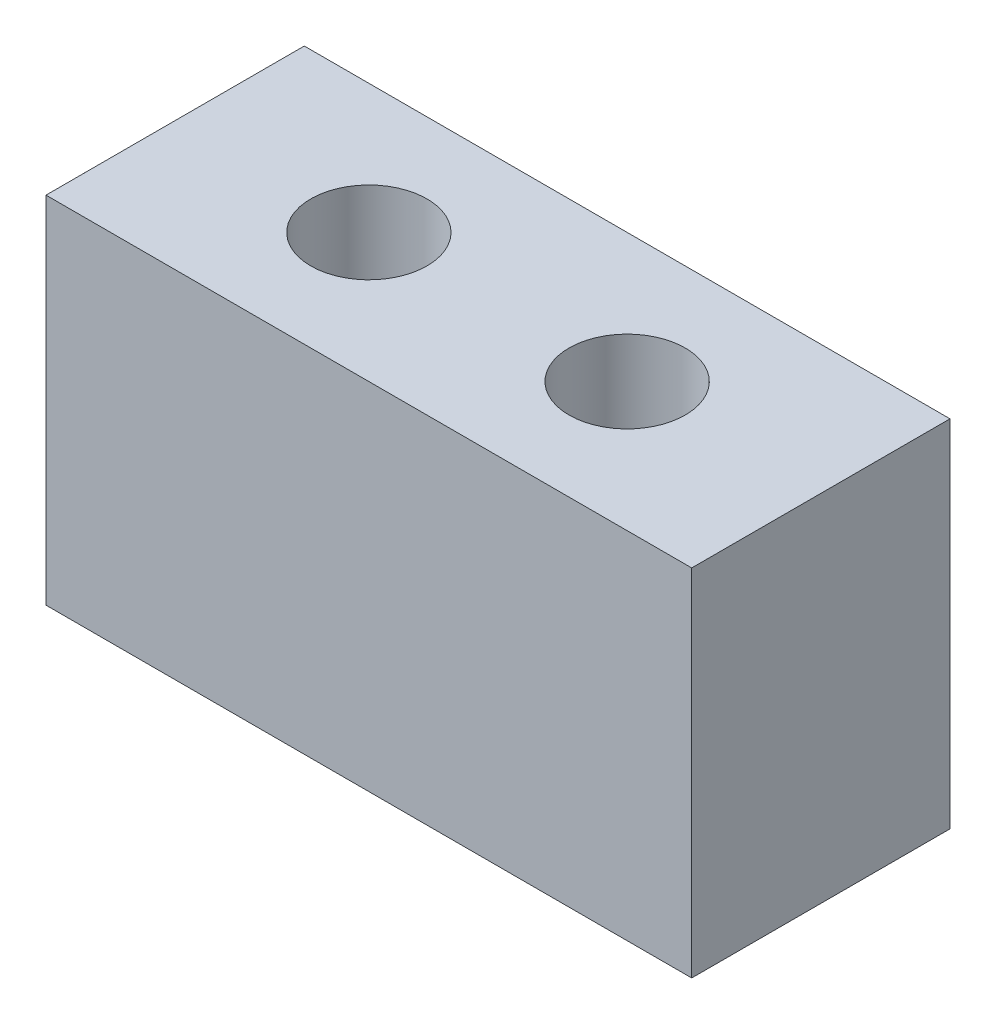
SolidWorks part; units mm, degrees
ref_plane "Front Plane" through (0, 0, 0) normal (0, 0, 1) x (1, 0, 0)
ref_plane "Top Plane" through (0, 0, 0) normal (0, 1, 0) x (1, 0, 0)
ref_plane "Right Plane" through (0, 0, 0) normal (1, 0, 0) x (0, 0, -1)
sketch "Sketch1" plane through (0, 0, 0) normal (0, 1, 0) x (1, 0, 0)
  line L1 (-50, -20) -> (50, -20)
  line L2 (-50, -20) -> (-50, 20)
  line L3 (-50, 20) -> (50, 20)
  line L4 (50, -20) -> (50, 20)
  line L5 (-50, -20) -> (50, 20) construction
  line L6 (-50, 20) -> (50, -20) construction
  circle A0 centre (-20, 0) radius 5.5
  circle A1 centre (20, 0) radius 5.5
  point P0 (0, 0)
  dimension "D3" = 11
  dimension "D4" = 11
  dimension "D1" = 40
  dimension "D2" = 100
  dimension "D5" = 20
  dimension "D6" = 20
extrude "Boss-Extrude1" add sketch "Sketch1" along normal blind 55
sketch "Sketch2" plane through (0, 55, 0) normal (0, 1, 0) x (1, 0, 0)
  circle A0 centre (20, 0) radius 9
  circle A1 centre (-20, 0) radius 9
  dimension "D1" = 18
  dimension "D2" = 18
extrude "Cut-Extrude1" cut sketch "Sketch2" against normal blind 20
